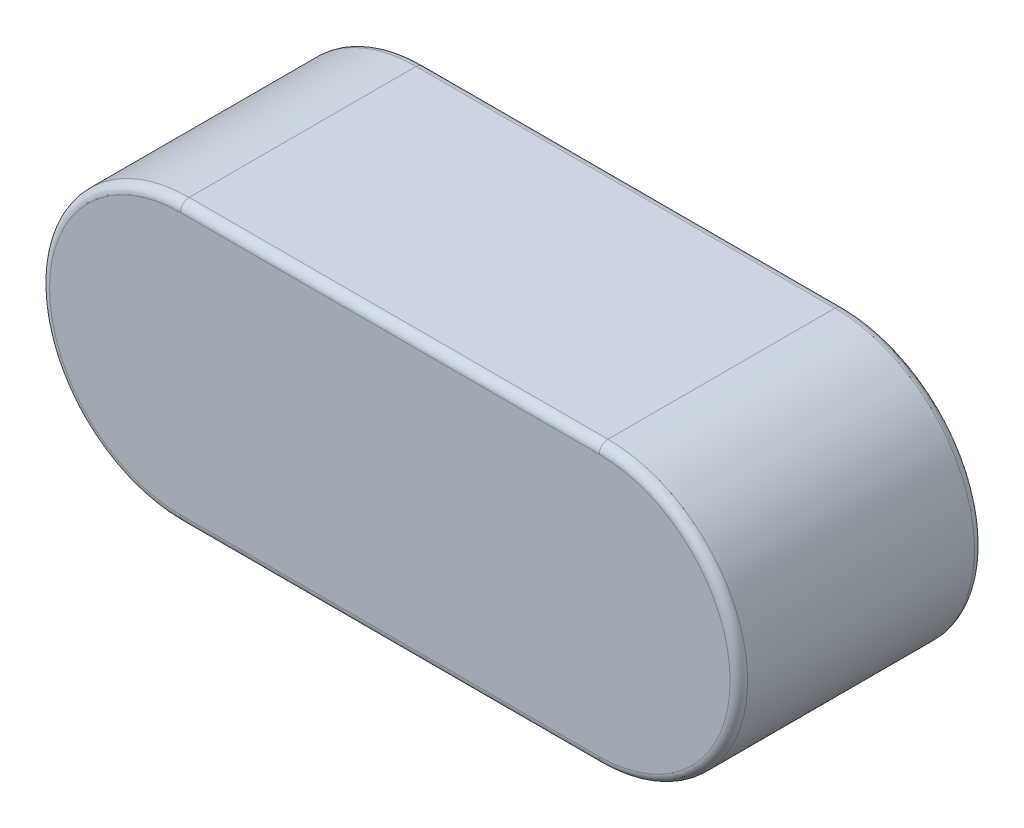
from build123d import *

# Parameters (mm, degrees)
EXTRUDE_487_DEPTH = 7
FILLET_1_R        = 0.25


with BuildPart() as part:
    # 草图1 → Extrude 487 (new body)
    with BuildSketch(Plane.XY):
        with BuildLine():
            Line((-6, 4), (6, 4))
            ThreePointArc((6, 4), (10, 0), (6, -4))
            Line((6, -4), (-6, -4))
            ThreePointArc((-6, -4), (-10, 0), (-6, 4))
        make_face()
    extrude(amount=EXTRUDE_487_DEPTH)

    # 圆角1
    fillet_1_edges = [part.edges().sort_by_distance(p)[0] for p in [
        (10, 0, 7),
        (0, 4, 7),
        (-10, 0, 7),
        (0, 4, 0),
        (10, 0, 0),
        (0, -4, 0),
        (-10, 0, 0),
        (0, -4, 7),
    ]]
    fillet(fillet_1_edges, radius=FILLET_1_R)


solid = part.part
